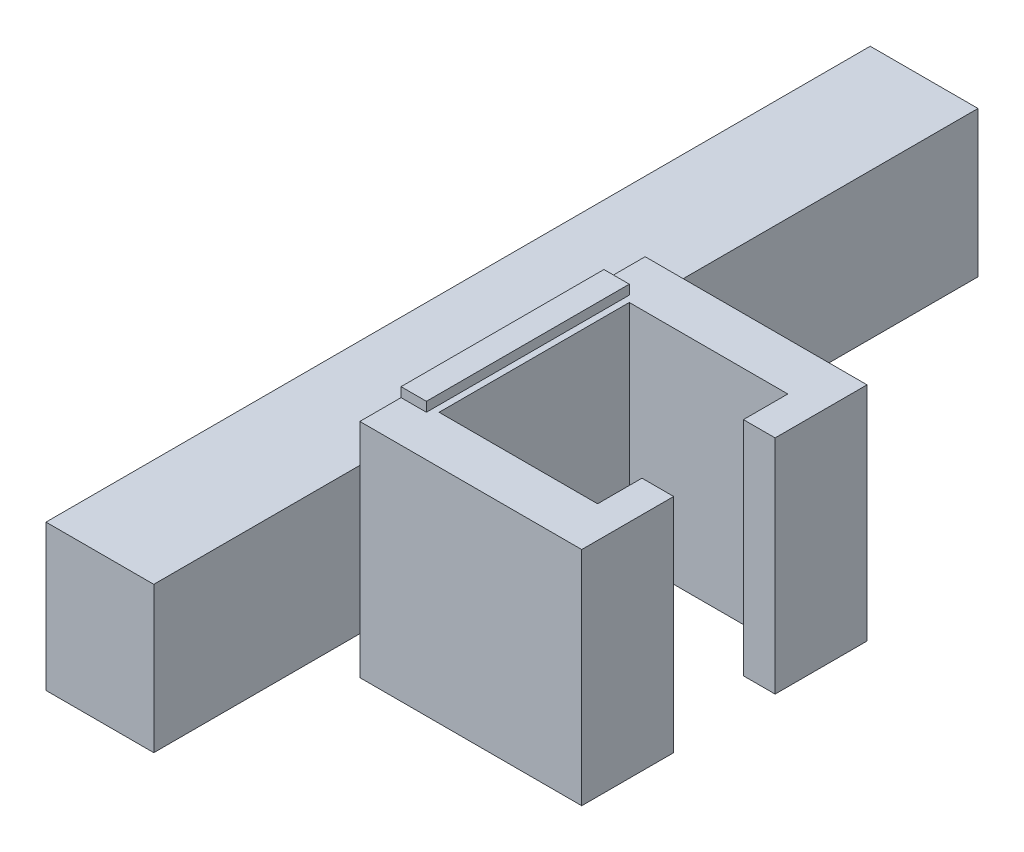
from build123d import *

# Parameters (mm, degrees)
BOSS_EXTRUDE1_DEPTH = 350
SKETCH2_W           = 320
SKETCH2_H           = 380
BOSS_EXTRUDE2_DEPTH = 40
SKETCH3_W           = 1500
SKETCH3_H           = 230
BOSS_EXTRUDE3_DEPTH = 170
SKETCH5_W           = 220.101814103
SKETCH5_H           = 309.079143209
CUT_EXTRUDE2_DEPTH  = 200
BOSS_EXTRUDE4_DEPTH = 1170


with BuildPart() as part:
    # Sketch1 → Boss-Extrude1 (new body)
    with BuildSketch(Plane(origin=(0, 0, 0), x_dir=(1, 0, 0), z_dir=(0, 1, 0))):
        Polygon((125, 80), (175, 80), (175, 225), (-175, 225), (-175, -225), (175, -225), (175, -80), (125, -80), (125, -150), (-125, -150), (-125, 150), (125, 150), align=None)
    extrude(amount=BOSS_EXTRUDE1_DEPTH)

    # Sketch2 → Boss-Extrude2 (add)
    with BuildSketch(Plane.ZY.offset(175)):
        with Locations((0, 175)):
            Rectangle(SKETCH2_W, SKETCH2_H)
    extrude(amount=-BOSS_EXTRUDE2_DEPTH)

    # Sketch3 → Boss-Extrude3 (add)
    with BuildSketch(Plane.ZY.offset(175)):
        with Locations((0, 175)):
            Rectangle(SKETCH3_W, SKETCH3_H)
    extrude(amount=BOSS_EXTRUDE3_DEPTH)

    # Sketch5 → Cut-Extrude2 (cut)
    with BuildSketch(Plane.XY.offset(750)):
        with Locations((-250.36904916, 177.341508661)):
            Rectangle(SKETCH5_W, SKETCH5_H)
    extrude(amount=-CUT_EXTRUDE2_DEPTH, mode=Mode.SUBTRACT)


with BuildPart() as body_2:
    # Sketch6 → Boss-Extrude4 (new body)
    with BuildSketch(Plane(origin=(0, 0, -735), x_dir=(-1, 0, 0), z_dir=(0, 0, -1))):
        Polygon((346, 215), (376, 215), (376, 200), (386, 200), (386, 215), (396, 215), (396, 135), (386, 135), (386, 150), (376, 150), (376, 135), (346, 135), align=None)
    extrude(amount=-BOSS_EXTRUDE4_DEPTH)


solid = Compound([part.part, body_2.part])
